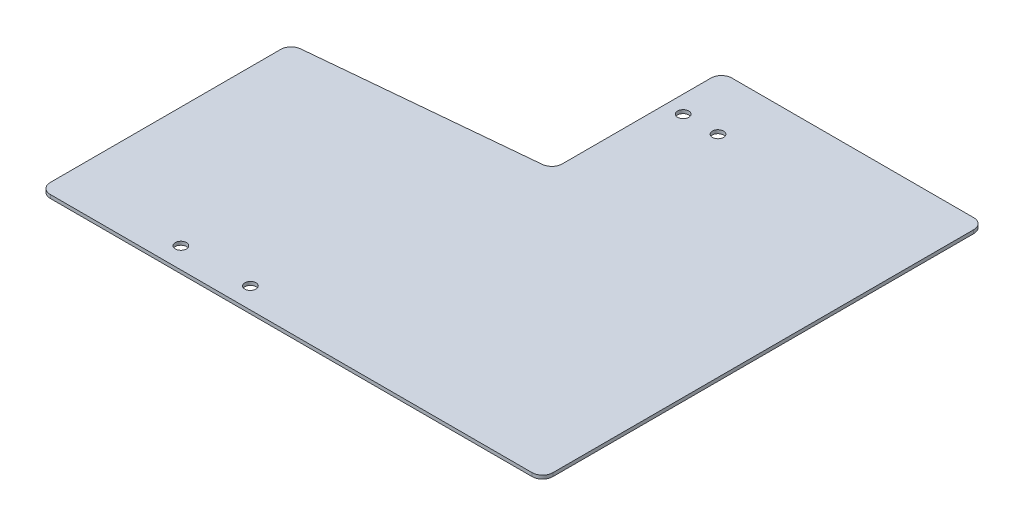
from build123d import *

# Parameters (mm, degrees)
SKETCH_1_R      = 1.6
EXTRUDE_1_DEPTH = 1
FILLET_1_R      = 3


with BuildPart() as part:
    # 草图1 → 凸台-拉伸1 (new body)
    with BuildSketch(Plane(origin=(0, 0, 0), x_dir=(1, 0, 0), z_dir=(0, 1, 0))):
        Polygon((0, 0), (0, 72), (69, 78.5), (69, 127), (144.55, 127), (144.55, 0), align=None)
        with Locations(Location((74, 111, 0), (0, 0, 270))):
            Circle(SKETCH_1_R, mode=Mode.SUBTRACT)
        with Locations(Location((84, 111, 0), (0, 0, 270))):
            Circle(SKETCH_1_R, mode=Mode.SUBTRACT)
        with Locations(Location((34.55, 6, 0), (0, 0, 270))):
            Circle(SKETCH_1_R, mode=Mode.SUBTRACT)
        with Locations(Location((54.55, 6, 0), (0, 0, 270))):
            Circle(SKETCH_1_R, mode=Mode.SUBTRACT)
    extrude(amount=EXTRUDE_1_DEPTH)

    # 圆角1
    fillet_1_edges = [part.edges().sort_by_distance(p)[0] for p in [
        (0, 0.5, 0),
        (0, 0.5, -72),
        (69, 0.5, -78.5),
        (69, 0.5, -127),
        (144.55, 0.5, -127),
        (144.55, 0.5, 0),
    ]]
    fillet(fillet_1_edges, radius=FILLET_1_R)


solid = part.part
